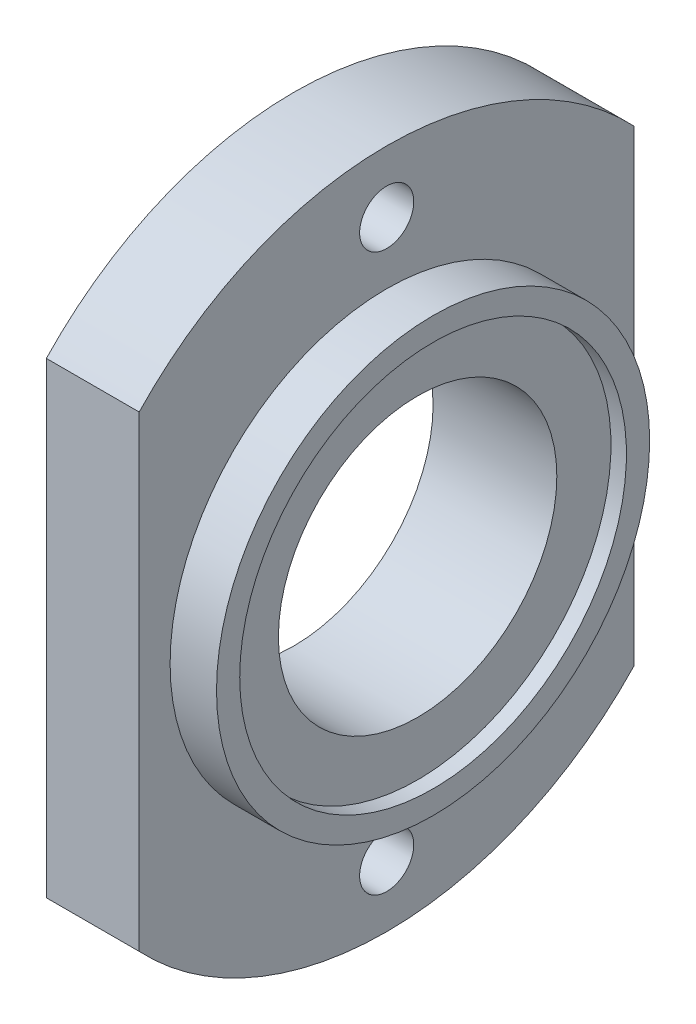
from build123d import *

# Parameters (mm, degrees)
SKETCH3_OUTSIDE_W                       = 58.574
SKETCH3_OUTSIDE_H                       = 58.574
SKETCH3_OUTSIDE_W_2                     = 32
SKETCH3_OUTSIDE_H_2                     = 50
CUT_EXTRUDE1_DEPTH                      = 33.388269481
CBORE_FOR_M3_HEX_HEAD_BOLT1_D           = 3.5
CBORE_FOR_M3_HEX_HEAD_BOLT1_CBORE_D     = 6
CBORE_FOR_M3_HEX_HEAD_BOLT1_CBORE_DEPTH = 3.5


with BuildPart() as part:
    # Sketch1 → Revolve1 (revolve)
    with BuildSketch(Plane.XY, mode=Mode.PRIVATE) as revolve1_sk:
        Polygon((0, 9), (0, 22), (6, 22), (6, 14), (9, 14), (9, 12.5), (8, 12.5), (8, 9), align=None)
    revolve(revolve1_sk.sketch.rotate(Axis((0, 0, 0), (1, 0, 0)), 90), axis=Axis((0, 0, 0), (1, 0, 0)))

    # Sketch3 outside → Cut-Extrude1 (cut, through all)
    with BuildSketch(Plane.ZY):
        Rectangle(SKETCH3_OUTSIDE_W, SKETCH3_OUTSIDE_H)
        Rectangle(SKETCH3_OUTSIDE_W_2, SKETCH3_OUTSIDE_H_2, mode=Mode.SUBTRACT)
    extrude(amount=-CUT_EXTRUDE1_DEPTH, mode=Mode.SUBTRACT)

    # CBORE for M3 Hex Head Bolt1 (through all)
    with Locations(Plane.ZY):
        with Locations((0, 18), (0, -18)):
            CounterBoreHole(CBORE_FOR_M3_HEX_HEAD_BOLT1_D / 2, CBORE_FOR_M3_HEX_HEAD_BOLT1_CBORE_D / 2, CBORE_FOR_M3_HEX_HEAD_BOLT1_CBORE_DEPTH)


solid = part.part
